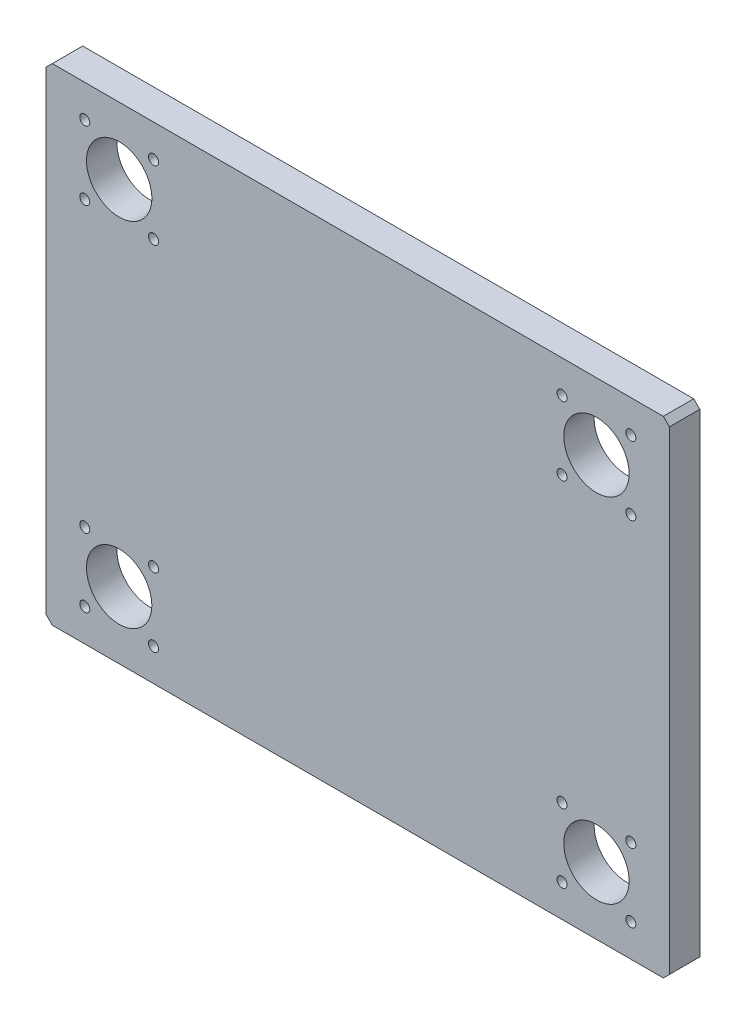
SolidWorks part; units mm, degrees
ref_plane "Front Plane" through (0, 0, 0) normal (0, 0, 1) x (1, 0, 0)
ref_plane "Top Plane" through (0, 0, 0) normal (0, 1, 0) x (1, 0, 0)
ref_plane "Right Plane" through (0, 0, 0) normal (1, 0, 0) x (0, 0, -1)
other "Configuration Table"
sketch "Sketch1" plane through (0, 0, 0) normal (0, 0, 1) x (1, 0, 0)
  line L1 (-102.5, -80) -> (102.5, -80)
  line L2 (-102.5, -80) -> (-102.5, 80)
  line L3 (-102.5, 80) -> (102.5, 80)
  line L4 (102.5, -80) -> (102.5, 80)
  line L5 (-102.5, -80) -> (102.5, 80) construction
  line L6 (-102.5, 80) -> (102.5, -80) construction
  point P0 (0, 0)
  dimension "D1" = 160
  dimension "D2" = 205
extrude "Boss-Extrude1" add sketch "Sketch1" along normal blind 10
sketch "Sketch2" plane through (0, 0, 10) normal (0, 0, 1) x (1, 0, 0)
  line L0 (-102.5, -80) -> (102.5, -80) construction
  line L1 (-102.5, 80) -> (-102.5, -80) construction
  line L2 (0, 0) -> (-102.5, 0) construction
  line L3 (0, 0) -> (0, 80) construction
  line L4 (102.5, 80) -> (-102.5, 80) construction
  circle A0 centre (-78.5, -58) radius 10.75
  circle A1 centre (-78.5, 58) radius 10.75
  circle A2 centre (78.5, -58) radius 10.75
  circle A3 centre (78.5, 58) radius 10.75
  dimension "D1" = 21.5
  dimension "D2" = 22
  dimension "D3" = 24
extrude "Cut-Extrude1" cut sketch "Sketch2" against normal through all
hole_wizard "M4 Tapped Hole1" positions "Sketch3" profile "Sketch4" tap size "M4" standard "GB" end condition through all
sketch "Sketch3" plane through (0, 0, 10) normal (0, 0, 1) x (1, 0, 0)
  point P0 (-89.8137, 69.3137)
  point P3 (-67.1863, 69.3137)
  point P6 (-67.1863, 46.6863)
  point P9 (-89.8137, 46.6863)
  point P12 (67.1863, 69.3137)
  point P15 (89.8137, 69.3137)
  point P18 (67.1863, 46.6863)
  point P21 (89.8137, 46.6863)
  point P24 (-89.8137, -46.6863)
  point P27 (-67.1863, -46.6863)
  point P30 (-89.8137, -69.3137)
  point P33 (-67.1863, -69.3137)
  point P36 (67.1863, -46.6863)
  point P39 (89.8137, -46.6863)
  point P42 (67.1863, -69.3137)
  point P45 (89.8137, -69.3137)
sketch "Sketch4" plane through (-89.8137, 69.3137, 10) normal (1, 0, 0) x (0, -1, 0)
  line L0 (0, 0) -> (0, 10)
  line L1 (0, 10) -> (1.65, 10)
  line L2 (1.65, 10) -> (1.65, 0)
  line L5 (1.65, 0) -> (0, 0)
  line L11 (0, -6.35) -> (0, 107.95) construction
  dimension "通孔螺纹孔钻头直径" = 3.3
  dimension "通孔螺纹孔钻头深度" = 10
cosmetic thread "Cosmetic Thread1" parameters "D2"=4
cosmetic thread "Cosmetic Thread2" parameters "D2"=4
cosmetic thread "Cosmetic Thread3" parameters "D2"=4
cosmetic thread "Cosmetic Thread4" parameters "D2"=4
cosmetic thread "Cosmetic Thread5" parameters "D2"=4
cosmetic thread "Cosmetic Thread6" parameters "D2"=4
cosmetic thread "Cosmetic Thread7" parameters "D2"=4
cosmetic thread "Cosmetic Thread8" parameters "D2"=4
cosmetic thread "Cosmetic Thread9" parameters "D2"=4
cosmetic thread "Cosmetic Thread10" parameters "D2"=4
cosmetic thread "Cosmetic Thread11" parameters "D2"=4
cosmetic thread "Cosmetic Thread12" parameters "D2"=4
cosmetic thread "Cosmetic Thread13" parameters "D2"=4
cosmetic thread "Cosmetic Thread14" parameters "D2"=4
cosmetic thread "Cosmetic Thread15" parameters "D2"=4
cosmetic thread "Cosmetic Thread16" parameters "D2"=4
chamfer "Chamfer1" distance 2 angle 45 4 edges at (-102.5, 80, 5) (102.5, 80, 5) (-102.5, -80, 5) (102.5, -80, 5)
